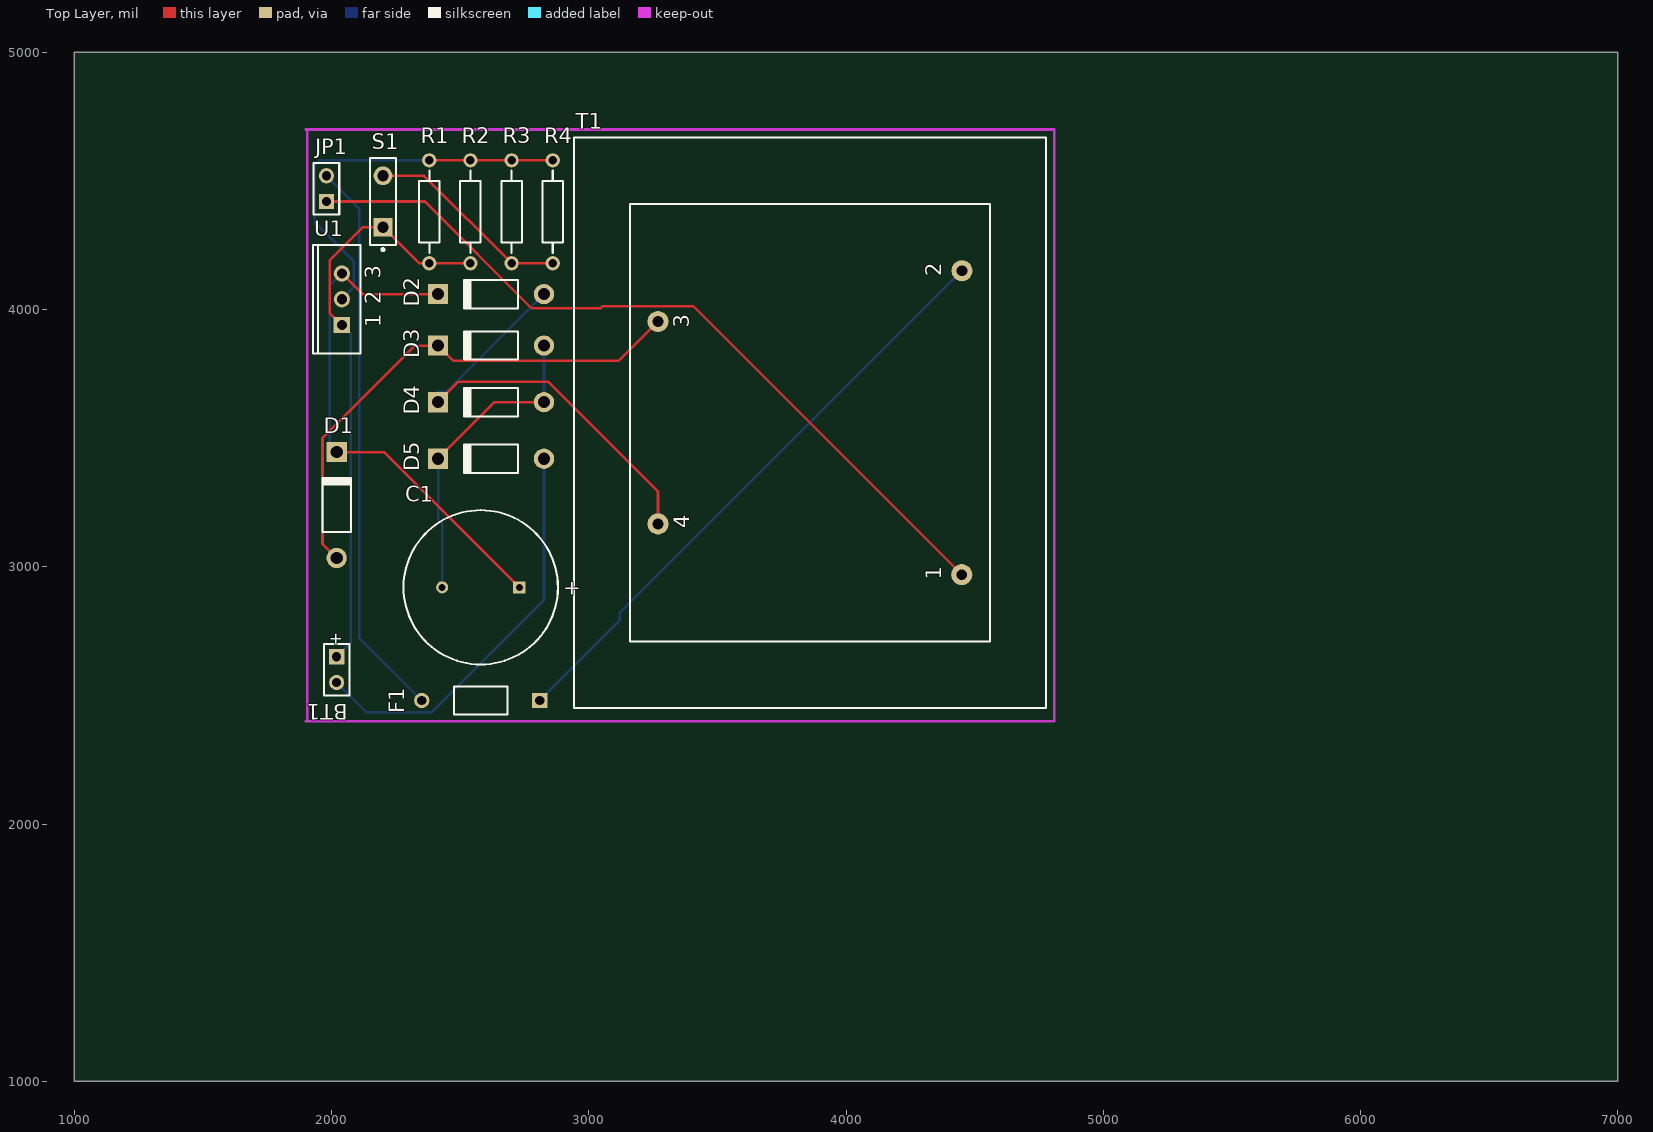
[diagram p0: Top Layer view]
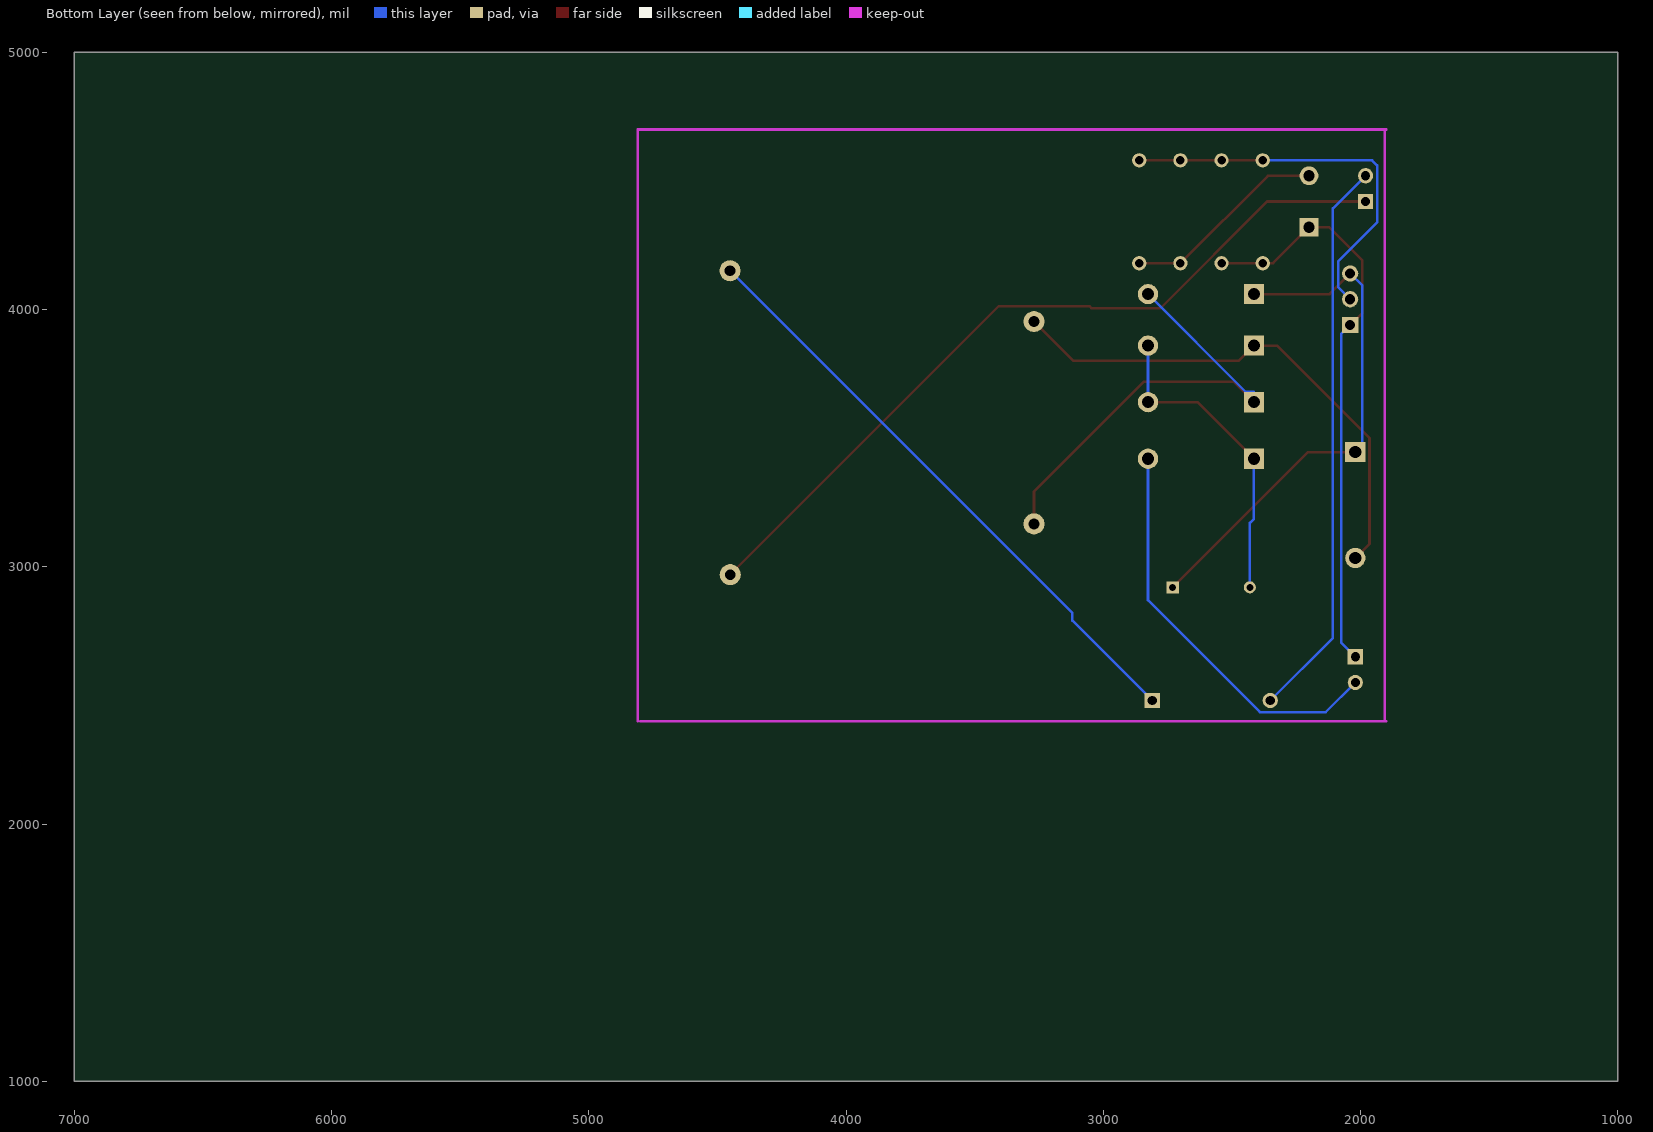
[diagram p1: Bottom Layer view, seen from below]
# Altium PCB MISC95143.PCBDOC
Units mil, origin at the board's own origin, x right, y up, seen from the top; angles counter-clockwise.
Board outline 6000 x 4000 mil, 2 copper layers (Top Layer, Bottom Layer); 16 components, 11 nets, 35 pads, 0 vias.

## Layer stack, top to bottom (the 12.6 mil dielectric is the usual default, probably not edited)
Top Layer: signal copper 1.4
Dielectric: dielectric 12.6, FR-4, Dk 4.8
Bottom Layer: signal copper 1.4

## Board outline
1000,1000 7000,1000 7000,5000 1000,5000

## Design rules (kind name [scope] priority, off if disabled: settings)
Clearance [All] p1: gap=10
ComponentClearance [All] p1: gap=10 collisioncheckmode=0
FanoutControl [All] p1: bgadir=Out bgaviamode=Centered fanoutstyle=Auto fanoutdirection=Alternating viagrid=1
PolygonConnect [All] p1: connectstyle=Relief reliefconductorwidth=10 reliefentries=4 polygonreliefangle="90 Angle"
RoutingCorners [All] p1: cornerstyle=Round minsetback=100 maxsetback=100
RoutingLayers [All] p1: top layer=Horizontal bottom layer=Vertical
RoutingVias [All] p1: holewidth=28 width=50 viastyle="Through Hole" minholewidth=28 minwidth=50 maxholewidth=28 maxwidth=50
SolderMaskExpansion [All] p1: expansion=4
TestPointUsage [All] p1: valid=0 allowmultiple=FALSE
Testpoint [All] p1: side=15 testpointundercomponent=TRUE minsize=40 maxsize=100 preferedsize=60 minholesize=0 maxholesize=40 preferedholesize=32 testpointgrid=1 style=1023 order=-539222988
Width Width_1 [All] p1: maxlimit=10 minlimit=10 preferedwidth=10
10 further rules are at their usual default settings.

## Components (designator, comment, footprint, x,y, rotation, side; value= is the part's Value field where it differs from the comment)
BT1 "Battery" BAT-2 2020,2600 r270 top
C1 "Cap Pol1" RB7.6-15 2580,2920 r0 top
D1 "Diode 1N4007" DIO10.46-5.3x2.8 2020,3240 r90 top
D2 "Diode 1N4007" DIO10.46-5.3x2.8 2620,4060 r180 top
D3 "Diode 1N4007" DIO10.46-5.3x2.8 2620,3860 r180 top
D4 "Diode 1N4007" DIO10.46-5.3x2.8 2620,3640 r180 top
D5 "Diode 1N4007" DIO10.46-5.3x2.8 2620,3420 r180 top
F1 "Fuse 1" PIN-W2/E2.8 2580,2480 r180 top
JP1 "Header 2" HDR1X2 1980,4420 r90 top
R1 "Res2" AXIAL-0.4 2380,4380 r90 top
R2 "Res2" AXIAL-0.4 2540,4380 r90 top
R3 "Res2" AXIAL-0.4 2700,4380 r90 top
R4 "Res2" AXIAL-0.4 2860,4380 r90 top
S1 "SW-PB" SPST-2 2200,4420 r90 top
T1 "Trans Cupl" TRF_4 3860,3560 r90 top
U1 "LM317KC" KC03 2040,4040 r90 top

## Footprints (in the part's own frame and the unit in brackets; to place one, negate y for a bottom-side part, rotate by r counter-clockwise, add the part's x,y. Pads: shape width x height; smd on the part's side, far side on the other; paste and mask are expansions set on the pad)
AXIAL-0.4 [mm]
  round 1.4 hole 0.85: 1(-5.08,0) 2(5.08,0)
  silkscreen extent -4.06,-1.02 4.06,1.02
BAT-2 [mm]
  rect 1.5x1.5 hole 0.9: 1(-1.27,0)
  round 1.5 hole 0.9: 2(1.27,0)
  silkscreen extent -2.54,-1.27 2.54,1.27
DIO10.46-5.3x2.8 [mm]
  round 2 hole 1.2: 1(-5.23,0)
  rect 2x2 hole 1.2: 2(5.23,0)
  silkscreen extent -2.65,-1.4 2.75,1.4
HDR1X2 [mm] "Connector; Header; 2 Position"
  rect 1.5x1.5 hole 0.9: 1(0,0)
  round 1.5 hole 0.9: 2(2.54,0)
  silkscreen extent -1.27,-1.27 3.81,1.27
KC03 [mm] "TO, Thru-Hole, Vertical, Heatsink Mounted; 3 In-Line Leads; Pitch 2.54 mm"
  rect 1.6x1.6 hole 1: 1(-2.54,0)
  round 1.6 hole 1: 2(0,0) 3(2.54,0)
  silkscreen extent -5.35,-1.85 5.35,2.85
PIN-W2/E2.8 [mm]
  rect 1.5x1.5 hole 0.9: 1(-5.825,0)
  round 1.5 hole 0.9: 2(5.825,0)
  silkscreen extent -2.65,-1.4 2.65,1.4
RB7.6-15 [mm]
  rect 1.2x1.2 hole 0.7: 1(3.81,0)
  round 1.2 hole 0.7: 2(-3.81,0)
  silkscreen extent -7.62,-7.62 7.62,7.62
SPST-2 [mm]
  rect 1.85x1.85 hole 1.1: 1(-2.54,0)
  round 1.85 hole 1.1: 2(2.54,0)
  silkscreen extent -4.89,-1.27 4.28,1.27
TRF_4 [mil]
  round 82 hole 42: 1(-590.83,-590) 2(590.83,-590.83) 3(393.33,590.83) 4(-393.33,590.83)
  silkscreen extent -1108,-917 1108,917

## Part data
BT1: "Multicell Battery"
C1: "Polarized Capacitor (Radial)"
D1 D2 D3 D4 D5: "1 Amp General Purpose Rectifier"
F1: "Fuse"
JP1: "Header, 2-Pin"
R1 R2 R3 R4: "Resistor"
S1: "Switch"
T1: "Transformer (Coupled Inductor Model)"
U1: "3-Terminal Adjustable Regulator"

## Nets (pads, with @x,y where several pads share a name; then routed paths per layer and width w, separated by ;. In a path a pad name is that pad's centre, name@x,y a point inside that pad or via, vN(x,y) a via of type N, cw(c..) or ccw(c..) an arc to the next point about the centre after c; other vN are vias at no path point)
NetBT1_1: BT1.1 R1.1 R2.1 S1.1 U1.1 | length 2256.2
  Top Layer w10: U1.1 1993,3987 1993,4191 2122,4320 S1.1 2340,4180 R1.1 R2.1
  Bottom Layer w10: BT1.1 2075,2705 2075,3905 U1.1
NetBT1_2: BT1.2 D5.1 | length 1583.8
  Bottom Layer w10: BT1.2 2135,2435 2391,2435 2825.91,2869.91 D5.1
NetC1_1: C1.1 D1.2 D2.2 U1.3 | length 2075.6
  Top Layer w10: D1.2 2204.09,3445.91 C1.1 ; U1.3 2120,4060 D2.2
  Bottom Layer w10: D1.2 1993,3445.91 1993,4093 U1.3
NetC1_2: C1.2 D3.1 D4.1 D5.2 | length 1229.5
  Top Layer w10: D5.2 2634.09,3640 D4.1
  Bottom Layer w10: D5.2 2414.09,3185.91 2430,3170 C1.2 ; D4.1 D3.1
NetD1_1: D1.1 D3.2 T1.3 | length 2029.5
  Top Layer w10: D1.1 1965,3089.09 1965,3500 2325,3860 D3.2 2473.09,3801 3116.83,3801 T1.3
NetD2_1: D2.1 D4.2 T1.4 | length 1799.9
  Top Layer w10: D4.2 2494.09,3720 2841,3720 3269.17,3291.83 T1.4
  Bottom Layer w10: D4.2 2414.09,3680 2445.91,3680 D2.1
NetF1_1: F1.1 T1.2 | length 2350.8
  Bottom Layer w10: F1.1 3120,2790.67 3120,2820 T1.2
NetF1_2: F1.2 JP1.2 | length 2193.5
  Bottom Layer w10: JP1.2 2107,4393 2107,2723.67 F1.2
NetJP1_1: JP1.1 T1.1 | length 3077.6
  Top Layer w10: JP1.1 2363,4420 2778,4005 3046,4005 3054,4013 3406.17,4013 T1.1
NetR1_2: R1.2 R2.2 R3.2 R4.2 U1.2 | length 1535.7
  Top Layer w10: R1.2 R2.2 R3.2 R4.2
  Bottom Layer w10: U1.2 2087,4087 2087,4186.5 1935,4338.5 1935,4560 1955,4580 R1.2
NetR3_1: R3.1 R4.1 S1.2 | length 800.8
  Top Layer w10: S1.2 2360,4520 R3.1 R4.1

## Keep-outs
Keep-Out Layer:
  lines w10: 1900,2400 4800,2400 ; 1900,4700 4810,4700 4810,2400 ; 1905,2400 1905,4700